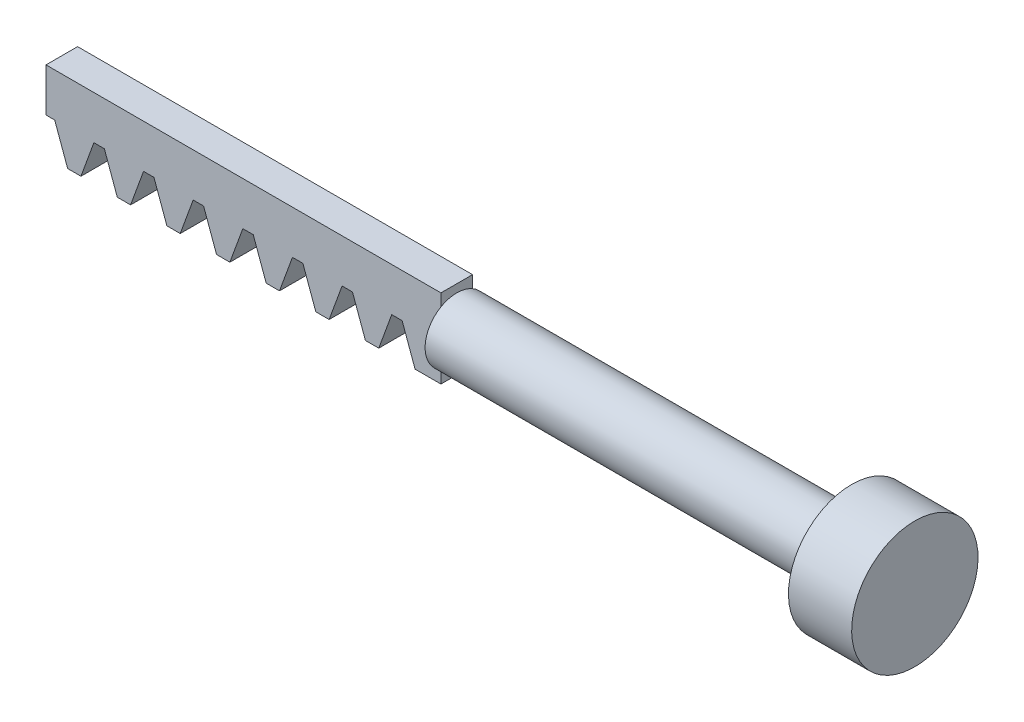
from build123d import *

# Parameters (mm, degrees)
SKETCH1_W           = 50
SKETCH1_H           = 10
BOSS_EXTRUDE1_DEPTH = 4
CUT_EXTRUDE1_DEPTH  = 52.14684741
CUT_EXTRUDE2_DEPTH  = 52.14684741
CUT_EXTRUDE3_DEPTH  = 52.14684741
CUT_EXTRUDE4_DEPTH  = 52.14684741
CUT_EXTRUDE5_DEPTH  = 52.14684741
CUT_EXTRUDE6_DEPTH  = 52.14684741
CUT_EXTRUDE7_DEPTH  = 52.14684741
CUT_EXTRUDE8_DEPTH  = 52.14684741


with BuildPart() as part:
    # Sketch1 → Boss-Extrude1 (new body)
    with BuildSketch(Plane.XY.offset(2)):
        with Locations((-25, 5)):
            Rectangle(SKETCH1_W, SKETCH1_H)
    extrude(amount=-BOSS_EXTRUDE1_DEPTH)

    # Sketch2 → Cut-Extrude1 (cut, through all)
    with BuildSketch(Plane(origin=(0, 0, -2), x_dir=(-1, 0, 0), z_dir=(0, 0, -1))):
        Polygon((40.976059531, 0), (45.573940469, 0), (43.936074414, 4.5), (42.613925586, 4.5), align=None)
    extrude(amount=-CUT_EXTRUDE1_DEPTH, mode=Mode.SUBTRACT)

    # Sketch3 → Cut-Extrude2 (cut, through all)
    with BuildSketch(Plane(origin=(0, 0, -2), x_dir=(-1, 0, 0), z_dir=(0, 0, -1))):
        Polygon((34.692059531, 0), (39.289940469, 0), (37.652074414, 4.5), (36.329925586, 4.5), align=None)
    extrude(amount=-CUT_EXTRUDE2_DEPTH, mode=Mode.SUBTRACT)

    # Sketch4 → Cut-Extrude3 (cut, through all)
    with BuildSketch(Plane(origin=(0, 0, -2), x_dir=(-1, 0, 0), z_dir=(0, 0, -1))):
        Polygon((28.408059531, 0), (33.005940469, 0), (31.368074414, 4.5), (30.045925586, 4.5), align=None)
    extrude(amount=-CUT_EXTRUDE3_DEPTH, mode=Mode.SUBTRACT)

    # Sketch5 → Cut-Extrude4 (cut, through all)
    with BuildSketch(Plane(origin=(0, 0, -2), x_dir=(-1, 0, 0), z_dir=(0, 0, -1))):
        Polygon((22.124059531, 0), (26.721940469, 0), (25.084074414, 4.5), (23.761925586, 4.5), align=None)
    extrude(amount=-CUT_EXTRUDE4_DEPTH, mode=Mode.SUBTRACT)

    # Sketch6 → Cut-Extrude5 (cut, through all)
    with BuildSketch(Plane(origin=(0, 0, -2), x_dir=(-1, 0, 0), z_dir=(0, 0, -1))):
        Polygon((15.840059531, 0), (20.437940469, 0), (18.800074414, 4.5), (17.477925586, 4.5), align=None)
    extrude(amount=-CUT_EXTRUDE5_DEPTH, mode=Mode.SUBTRACT)

    # Sketch7 → Cut-Extrude6 (cut, through all)
    with BuildSketch(Plane(origin=(0, 0, -2), x_dir=(-1, 0, 0), z_dir=(0, 0, -1))):
        Polygon((9.556059531, 0), (14.153940469, 0), (12.516074414, 4.5), (11.193925586, 4.5), align=None)
    extrude(amount=-CUT_EXTRUDE6_DEPTH, mode=Mode.SUBTRACT)

    # Sketch8 → Cut-Extrude7 (cut, through all)
    with BuildSketch(Plane(origin=(0, 0, -2), x_dir=(-1, 0, 0), z_dir=(0, 0, -1))):
        Polygon((3.272059531, 0), (7.869940469, 0), (6.232074414, 4.5), (4.909925586, 4.5), align=None)
    extrude(amount=-CUT_EXTRUDE7_DEPTH, mode=Mode.SUBTRACT)

    # Sketch9 → Cut-Extrude8 (cut, through all)
    with BuildSketch(Plane(origin=(0, 0, -2), x_dir=(-1, 0, 0), z_dir=(0, 0, -1))):
        Polygon((48.897925586, 4.5), (47.260059531, 0), (50, 0), (50, 4.5), align=None)
    extrude(amount=-CUT_EXTRUDE8_DEPTH, mode=Mode.SUBTRACT)

    # Sketch10 → Revolve1 (revolve)
    with BuildSketch(Plane.XY):
        Polygon((0, 9), (0, 5), (58, 5), (58, 13), (50, 13), (50, 9), align=None)
    revolve(axis=Axis((0, 5, 0), (1, 0, 0)))


solid = part.part
